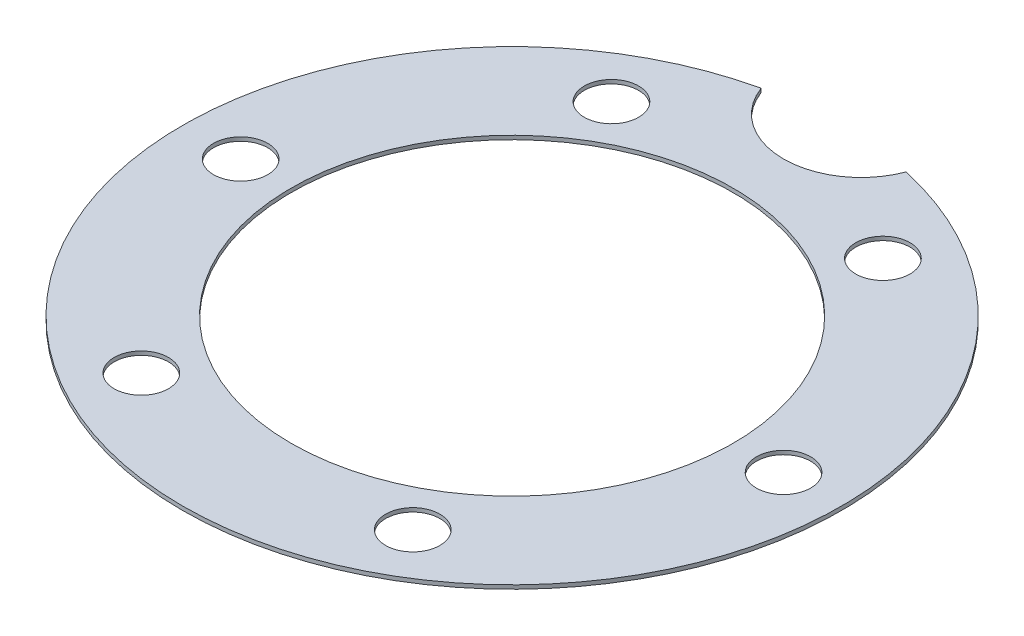
from build123d import *

# Parameters (mm, degrees)
SKETCH1_R           = 7
SKETCH1_R_2         = 57
BOSS_EXTRUDE1_DEPTH = 1


with BuildPart() as part:
    # Sketch1 → Boss-Extrude1 (new body)
    with BuildSketch(Plane(origin=(0, 0, 0), x_dir=(1, 0, 0), z_dir=(0, 1, 0))):
        with BuildLine():
            ThreePointArc((-18.703646406, 82.916666667), (0, -85), (18.703646406, 82.916666667))
            ThreePointArc((18.703646406, 82.916666667), (0, 70), (-18.703646406, 82.916666667))
        make_face()
        with Locations(Location((-35, 60.621778265, 0), (0, 0, 270))):
            Circle(SKETCH1_R, mode=Mode.SUBTRACT)
        with Locations(Location((35, 60.621778265, 0), (0, 0, 270))):
            Circle(SKETCH1_R, mode=Mode.SUBTRACT)
        with Locations(Location((70, 0, 0), (0, 0, 270))):
            Circle(SKETCH1_R, mode=Mode.SUBTRACT)
        with Locations(Location((35, -60.621778265, 0), (0, 0, 270))):
            Circle(SKETCH1_R, mode=Mode.SUBTRACT)
        with Locations(Location((-35, -60.621778265, 0), (0, 0, 270))):
            Circle(SKETCH1_R, mode=Mode.SUBTRACT)
        with Locations(Location((-70, 0, 0), (0, 0, 270))):
            Circle(SKETCH1_R, mode=Mode.SUBTRACT)
        with Locations(Location((0, 0, 0), (0, 0, 270))):
            Circle(SKETCH1_R_2, mode=Mode.SUBTRACT)
    extrude(amount=BOSS_EXTRUDE1_DEPTH)


solid = part.part
